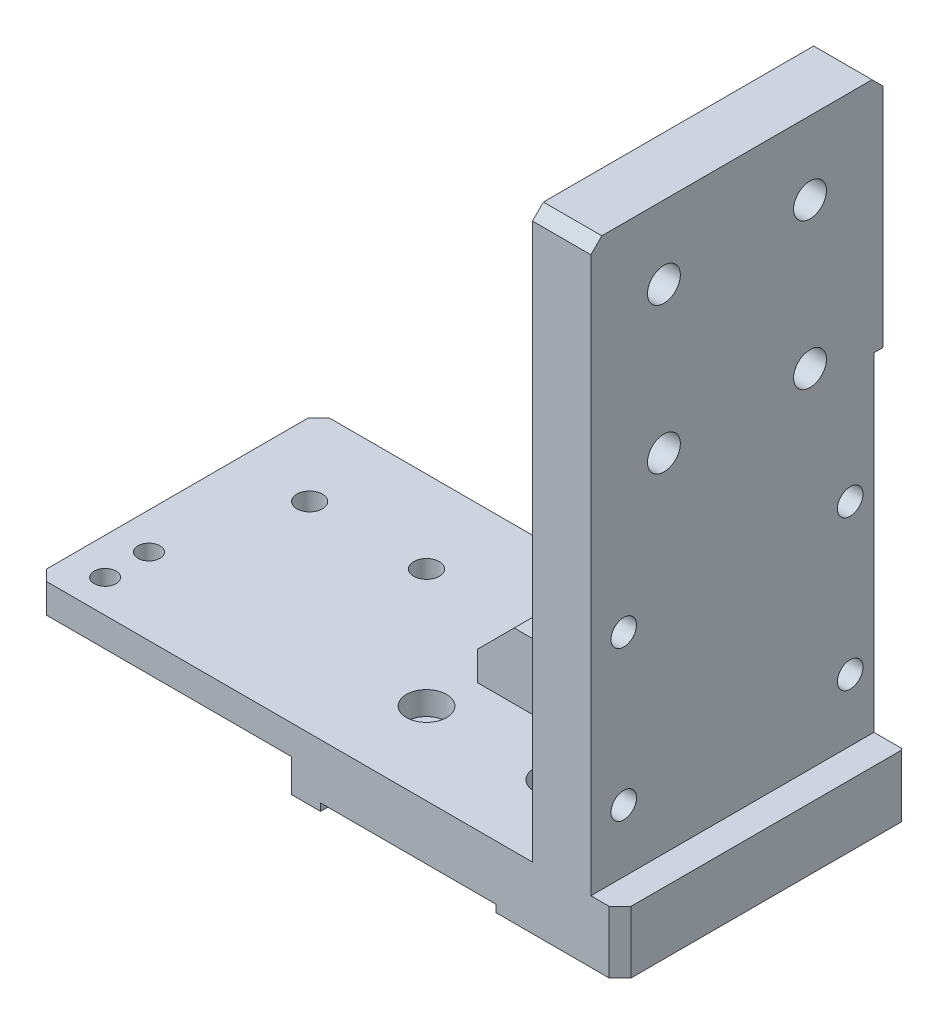
SolidWorks part; units mm, degrees
ref_plane "前视基准面" through (0, 0, 0) normal (0, 0, 1) x (1, 0, 0)
ref_plane "上视基准面" through (0, 0, 0) normal (0, 1, 0) x (1, 0, 0)
ref_plane "右视基准面" through (0, 0, 0) normal (1, 0, 0) x (0, 0, -1)
sketch "草图2" plane through (0, 0, 0) normal (0, 0, 1) x (1, 0, 0)
  line L0 (46, -8.5) -> (80, -8.5)
  line L1 (-80, 8.5) -> (56, 8.5)
  line L2 (-80, 8.5) -> (-80, -8.5)
  line L3 (-80, -8.5) -> (-2, -8.5)
  line L4 (80, 8.5) -> (80, -8.5)
  line L5 (-80, 8.5) -> (80, -8.5) construction
  line L6 (-80, -8.5) -> (80, 8.5) construction
  line L8 (56, 8.5) -> (56, 163.5)
  line L9 (56, 163.5) -> (72, 163.5)
  line L10 (72, 8.5) -> (72, 163.5)
  line L11 (72, 8.5) -> (80, 8.5)
  line L12 (-2, -8.5) -> (-2, -6.5)
  line L13 (-2, -6.5) -> (46, -6.5)
  line L14 (46, -8.5) -> (46, -6.5)
  point P0 (0, 0)
  dimension "D1" = 160
  dimension "D2" = 17
  dimension "D3" = 8
  dimension "D4" = 16
  dimension "D5" = 172
  dimension "D6" = 2
  dimension "D7" = 48
  dimension "D8" = 34
extrude "凸台-拉伸2" add sketch "草图2" along normal mid plane 80
sketch "草图4" plane through (56, 0, 0) normal (-1, 0, 0) x (0, 0, 1)
  line L1 (-40, 8.5) -> (-37.5, 8.5)
  line L2 (-40, 8.5) -> (-40, 98.5)
  line L3 (-40, 98.5) -> (-37.5, 98.5)
  line L4 (-37.5, 8.5) -> (-37.5, 98.5)
  dimension "D1" = 90
  dimension "D2" = 2.5
extrude "切除-拉伸2" cut sketch "草图4" against normal blind 80
sketch "草图5" plane through (0, 0, 0) normal (0, 0, 1) x (1, 0, 0)
  line L0 (46, 8.5) -> (6, 8.5)
  line L1 (56, 8.5) -> (-80, 8.5) construction
  line L2 (6, 8.5) -> (6, 26.5)
  line L3 (6, 26.5) -> (38, 26.5)
  line L4 (38, 26.5) -> (38, 83.5)
  line L5 (38, 83.5) -> (56, 83.5)
  line L6 (56, 163.5) -> (56, 8.5) construction
  line L7 (56, 83.5) -> (56, 18.5)
  line L8 (46, 8.5) -> (56, 18.5)
  dimension "D1" = 50
  dimension "D2" = 18
  dimension "D3" = 18
  dimension "D4" = 75
  dimension "D5" = 10
  dimension "D6" = 10
extrude "凸台-拉伸3" add sketch "草图5" along normal mid plane 10 contours L4 L5 L7 L8 L0 L2 L3
fillet "圆角1" radius 10 1 edges at (38, 26.5, 0)
chamfer "倒角1" distance 10 angle 45 2 edges at (6, 26.5, 0) (38, 83.5, 0)
hole_wizard "M6 六角凹头螺钉的柱形沉头孔1" positions "草图7" profile "草图6" counterbore size "M6" standard "ISO" end condition through all
sketch "草图7" plane through (0, 8.5, 0) normal (0, 1, 0) x (1, 0, 0)
  line L1 (0, 0) -> (30.9339, 0) construction
  line L2 (80, -40) -> (80, 40) construction
  point P0 (4.5, 17.5)
  point P2 (39.5, 17.5)
  point P12 (39.5, -17.5)
  point P13 (4.5, -17.5)
  dimension "D1" = 40.5
  dimension "D2" = 35
  dimension "D3" = 17.5
sketch "草图6" plane through (4.5, 8.5, -17.5) normal (1, 0, 0) x (0, 0, 1)
  line L0 (0, 0) -> (0, 17)
  line L1 (0, 17) -> (3.3, 17)
  line L3 (3.3, 17) -> (3.3, 6.4)
  line L4 (3.3, 6.4) -> (5.5, 6.4)
  line L5 (5.5, 6.4) -> (5.5, 0)
  line L7 (5.5, 0) -> (0, 0)
  line L11 (0, -6.35) -> (0, 107.95) construction
  dimension "通孔孔直径" = 6.6
  dimension "通孔孔深度" = 17
  dimension "柱形沉头孔直径" = 11
  dimension "柱形沉头孔深度" = 6.4
hole_wizard "Ø12.0 (12) 直径孔1" positions "草图9" profile "草图8" hole size "Ø12.0" standard "ISO"
sketch "草图9" plane through (0, 8.5, 0) normal (0, 1, 0) x (1, 0, 0)
  line L0 (-80, -40) -> (-80, 40) construction
  point P0 (-65.5, 25)
  point P2 (-40.5, 25)
  point P14 (-65.5, -25)
  point P15 (-40.5, -25)
  dimension "D1" = 14.5
  dimension "D2" = 25
  dimension "D3" = 25
sketch "草图8" plane through (-65.5, 8.5, -25) normal (1, 0, 0) x (0, 0, 1)
  line L0 (0, 0) -> (0, 17)
  line L1 (0, 17) -> (6, 17)
  line L2 (6, 17) -> (6, 0)
  line L5 (6, 0) -> (0, 0)
  line L11 (0, -6.35) -> (0, 107.95) construction
  dimension "通孔孔直径" = 12
  dimension "通孔孔深度" = 17
hole_wizard "M8 六角凹头螺钉的柱形沉头孔1" positions "草图11" profile "草图10" counterbore size "M8" standard "ISO"
sketch "草图11" plane through (0, 8.5, 0) normal (0, 1, 0) x (1, 0, 0)
  line L0 (-80, -40) -> (-80, 40) construction
  point P0 (-65.5, 0)
  point P2 (-40.5, 0)
  dimension "D1" = 14.5
  dimension "D2" = 25
sketch "草图10" plane through (-65.5, 8.5, 0) normal (1, 0, 0) x (0, 0, 1)
  line L0 (0, 0) -> (0, 17)
  line L1 (0, 17) -> (4.5, 17)
  line L3 (4.5, 17) -> (4.5, 8.6)
  line L4 (4.5, 8.6) -> (7.5, 8.6)
  line L5 (7.5, 8.6) -> (7.5, 0)
  line L7 (7.5, 0) -> (0, 0)
  line L11 (0, -6.35) -> (0, 107.95) construction
  dimension "通孔孔直径" = 9
  dimension "通孔孔深度" = 17
  dimension "柱形沉头孔直径" = 15
  dimension "柱形沉头孔深度" = 8.6
chamfer "倒角2" distance 3 angle 45 5 edges at (64, 163.5, -40) (64, 163.5, 40) (80, 0, 40) (80, 0, -40) (-80, 0, 40)
hole_wizard "Ø7.0 (7) 直径孔1" positions "草图13" profile "草图12" hole size "Ø7.0" standard "ISO" end condition through all
sketch "草图13" plane through (56, 0, 0) normal (-1, 0, 0) x (0, 0, 1)
  line L0 (37, 163.5) -> (-37, 163.5) construction
  line L1 (-40, 160.5) -> (-40, 98.5) construction
  line L2 (0, 0) -> (0, 132.8924) construction
  point P0 (-31, 25.5)
  point P2 (-31, 66.5)
  point P15 (31, 66.5)
  point P16 (31, 25.5)
  dimension "D1" = 97
  dimension "D2" = 41
  dimension "D3" = 9
sketch "草图12" plane through (56, 25.5, -31) normal (0, 1, 0) x (0, 0, 1)
  line L0 (0, 0) -> (0, 24)
  line L1 (0, 24) -> (3.5, 24)
  line L2 (3.5, 24) -> (3.5, 0)
  line L5 (3.5, 0) -> (0, 0)
  line L11 (0, -6.35) -> (0, 107.95) construction
  dimension "通孔孔直径" = 7
  dimension "通孔孔深度" = 24
hole_wizard "M8 六角凹头螺钉的柱形沉头孔2" positions "草图15" profile "草图14" counterbore size "M8" standard "ISO" end condition through all
sketch "草图15" plane through (56, 0, 0) normal (-1, 0, 0) x (0, 0, 1)
  line L0 (37, 163.5) -> (-37, 163.5) construction
  line L1 (0, 0) -> (0, 202.2708) construction
  point P0 (-20, 143.5)
  point P2 (-20, 103.5)
  point P12 (20, 103.5)
  point P13 (20, 143.5)
  dimension "D1" = 20
  dimension "D2" = 20
  dimension "D3" = 40
sketch "草图14" plane through (56, 143.5, -20) normal (0, 1, 0) x (0, 0, 1)
  line L0 (0, 0) -> (0, 24)
  line L1 (0, 24) -> (4.5, 24)
  line L3 (4.5, 24) -> (4.5, 8.6)
  line L4 (4.5, 8.6) -> (7.5, 8.6)
  line L5 (7.5, 8.6) -> (7.5, 0)
  line L7 (7.5, 0) -> (0, 0)
  line L11 (0, -6.35) -> (0, 107.95) construction
  dimension "通孔孔直径" = 9
  dimension "通孔孔深度" = 24
  dimension "柱形沉头孔直径" = 15
  dimension "柱形沉头孔深度" = 8.6
sketch "草图16" plane through (0, 8.5, 0) normal (0, 1, 0) x (1, 0, 0)
  line L1 (80, -37) -> (80, 37) construction
  line L2 (80, 37.5) -> (-83.7116, 37.5)
  line L3 (80, 37.5) -> (80, 40)
  line L4 (80, 40) -> (-83.7116, 40)
  line L7 (-83.7116, 37.5) -> (-83.7116, 40)
  line L8 (77, 40) -> (-80, 40) construction
  dimension "D1" = 2.5
extrude "切除-拉伸3" cut sketch "草图16" against normal through all
sketch "草图17" plane through (0, 0, -37.5) normal (0, 0, -1) x (-1, 0, 0)
  line L0 (80, 8.5) -> (80, -8.5) construction
  line L1 (80, -8.5) -> (10, -8.5)
  line L2 (80, -8.5) -> (80, 0.5)
  line L3 (80, 0.5) -> (10, 0.5)
  line L4 (10, -8.5) -> (10, 0.5)
  dimension "D1" = 70
  dimension "D2" = 9
extrude "切除-拉伸4" cut sketch "草图17" against normal through all
chamfer "倒角4" distance 3 angle 45 1 edges at (-80, 4.5, -37.5)
hole_wizard "Ø7.0 (7) 直径孔2" positions "草图19" profile "草图20" hole size "Ø7.0" standard "GB" end condition through all
sketch "草图19" plane through (0, 8.5, 0) normal (0, 1, 0) x (1, 0, 0)
  point P0 (-28, 15)
  point P3 (-60, 15)
sketch "草图20" plane through (-28, 8.5, -15) normal (1, 0, 0) x (0, 0, 1)
  line L0 (0, 0) -> (0, 17)
  line L1 (0, 17) -> (3.5, 17)
  line L2 (3.5, 17) -> (3.5, 0)
  line L5 (3.5, 0) -> (0, 0)
  line L11 (0, -6.35) -> (0, 107.95) construction
  dimension "通孔孔直径" = 7
  dimension "通孔孔深度" = 17
hole_wizard "Ø6.0 (6) 直径孔1" positions "草图22" profile "草图21" hole size "Ø6.0" standard "GB" end condition through all
sketch "草图22" plane through (0, 8.5, 0) normal (0, 1, 0) x (1, 0, 0)
  point P0 (-70, -31)
  point P3 (-70, -19)
sketch "草图21" plane through (-70, 8.5, 31) normal (1, 0, 0) x (0, 0, 1)
  line L0 (0, 0) -> (0, 17)
  line L1 (0, 17) -> (3, 17)
  line L2 (3, 17) -> (3, 0)
  line L5 (3, 0) -> (0, 0)
  line L11 (0, -6.35) -> (0, 107.95) construction
  dimension "通孔孔直径" = 6
  dimension "通孔孔深度" = 17
